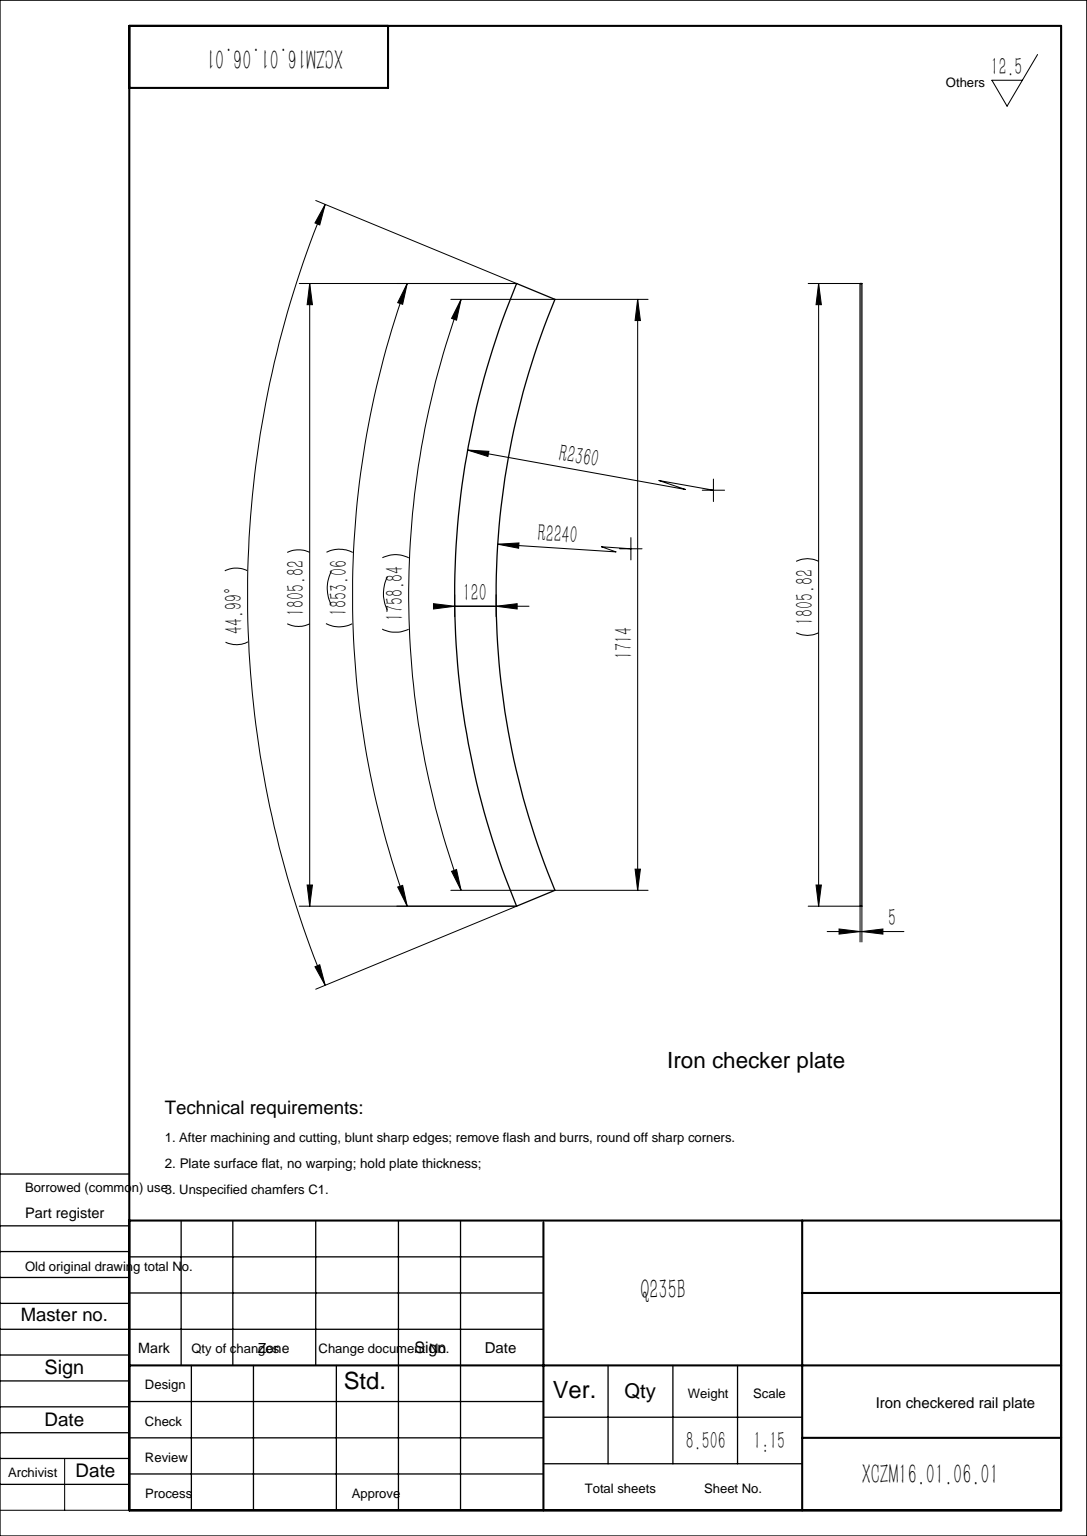
SolidWorks part; units mm, degrees
material "Q235B"
ref_plane "Front Plane" through (0, 0, 0) normal (0, 0, 1) x (1, 0, 0)
ref_plane "Top Plane" through (0, 0, 0) normal (0, 1, 0) x (1, 0, 0)
ref_plane "Right Plane" through (0, 0, 0) normal (1, 0, 0) x (0, 0, -1)
sketch "Sketch2" plane through (0, 0, 0) normal (0, 1, 0) x (1, 0, 0)
  line L0 (0, 0) -> (-902.9107, 2180.4477)
  line L1 (0, 2360) -> (0, 0) construction
  line L2 (0, 0) -> (902.9107, 2180.4477)
  line L3 (-902.9107, 2180.4477) -> (902.9107, 2180.4477) construction
  line L4 (-857, 2069.5775) -> (857, 2069.5775) construction
  circle A0 centre (0, 0) radius 2360
  circle A1 centre (0, 0) radius 2240
  dimension "D1" = 4720
  dimension "D2" = 4480
  dimension "D3" = 1714
  dimension "D4" = 1805.8214
  dimension "D5" = 1714
extrude "Boss-Extrude1" add sketch "Sketch2" along normal blind 5 contours A1 L2 A0 L0
